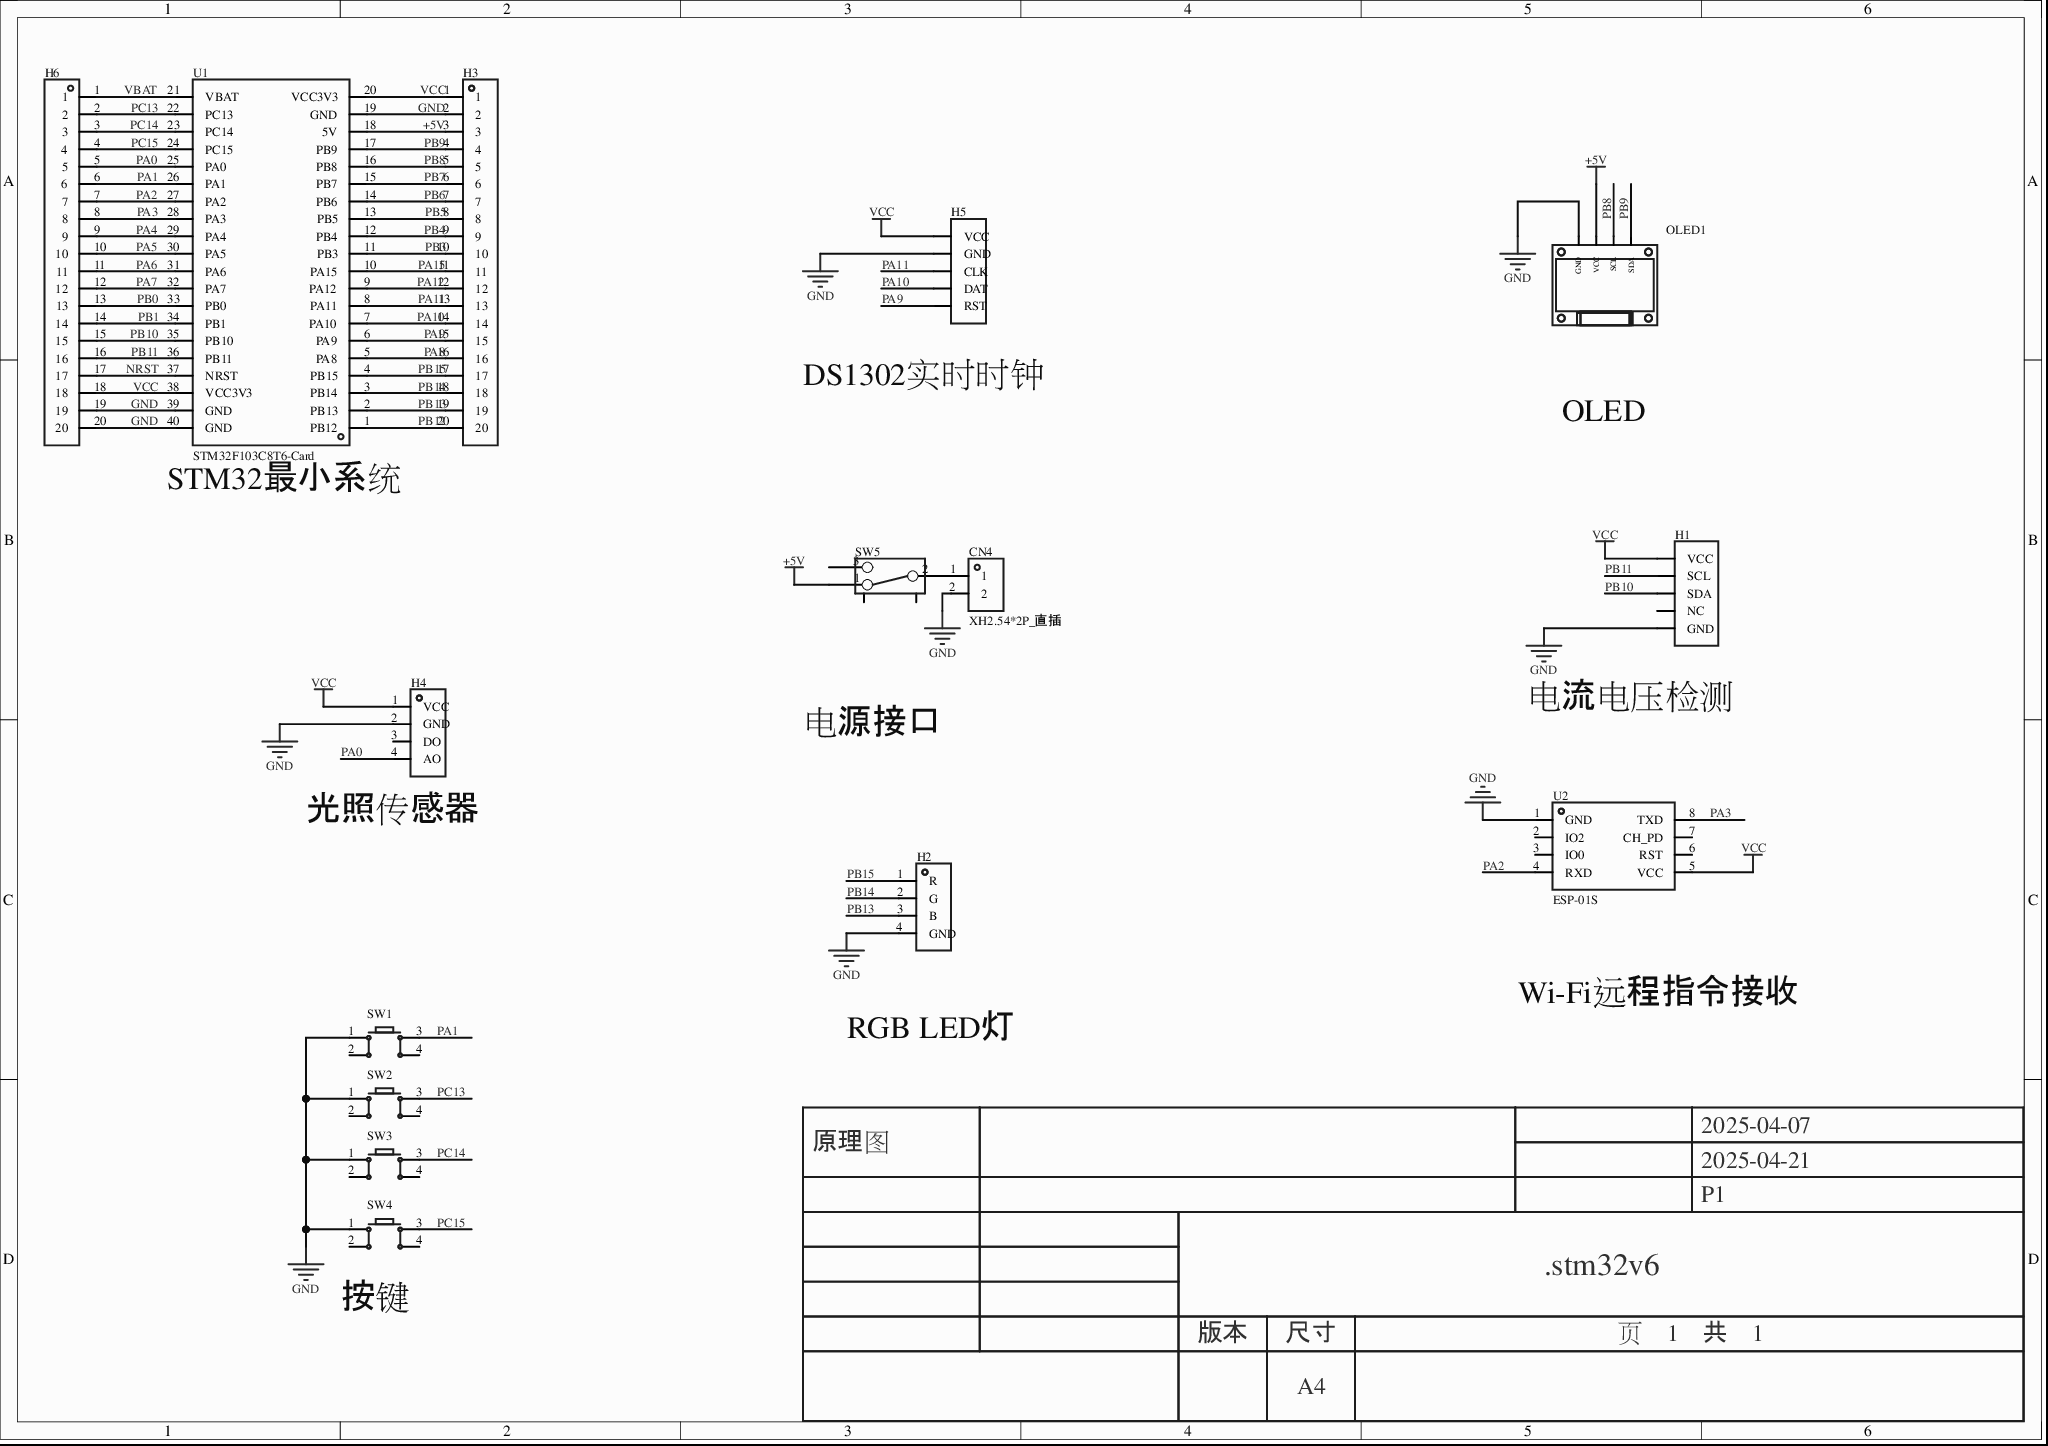
[diagram p0: MISC51840-3.schdoc]
# Altium project MISC51840-2.PrjPcb
1 sheet, 15 parts. Net scope: global (net labels, ports and power ports of the same name join across sheets).
Board file: MISC51840.pcbdoc

## Sheet MISC51840-3.schdoc
size 297 x 209 mm; Version: V1.0; @Project Name: MISC51840; @Page Count: 1; @Update Date: 2026-05-15; @Create Date: 2026-05-15; @Schematic Name: MISC51840; @Page No: 1; @Create Time: 23:22:16; @Update Time: 17:32:40; @Board Name: MISC51840

### Parts
CN4  XH2.54*2P_直插  [CONN-TH_2P-P2.50-XH2.54-2P]
H1  (no value)  [HDR-TH_5P-P2.54-V-F]
H2  (no value)  [HDR-TH_4P-P2.54-V-F]
H3  (no value)  [HDR-TH_20P-P2.54-V-M-1]
H4  (no value)  [HDR-TH_4P-P2.54-V-F]
H5  (no value)  [HDR-TH_5P-P2.54-V-F]
H6  (no value)  [HDR-TH_20P-P2.54-V-M-1]
OLED1  (no value)  [0.96OLED_4P]
SW1  (no value)  [SW-TH_4P-L6.0-W6.0-P4.50-LS6.5]
SW2  (no value)  [SW-TH_4P-L6.0-W6.0-P4.50-LS6.5]
SW3  (no value)  [SW-TH_4P-L6.0-W6.0-P4.50-LS6.5]
SW4  (no value)  [SW-TH_4P-L6.0-W6.0-P4.50-LS6.5]
SW5  (no value)  [拨动开关]
U1  STM32F103C8T6-Card  [CONN-TH_L53.3-W22.9_STM32F103C8T6-CARD]
U2  ESP-01S  [WIFIM-TH_ESP-01S]

### Nets
+5V: H3.3 OLED1.2(VCC) SW5.1 U1.18(5V)
GND: CN4.2 H1.5(GND) H2.4(GND) H3.2 H4.2(GND) H5.2(GND) H6.19 H6.20 OLED1.1(GND) SW1.1 SW2.1 SW3.1 SW4.1 U1.19(GND) U1.39(GND) U1.40(GND) U2.1(GND)
VCC: H1.1(VCC) H3.1 H4.1(VCC) H5.1(VCC) H6.18 U1.20(VCC3V3) U1.38(VCC3V3) U2.5(VCC)
NRST: H6.17 U1.37(NRST)
PA0: H4.4(AO) H6.5 U1.25(PA0)
PA1: H6.6 SW1.3 U1.26(PA1)
PA2: H6.7 U1.27(PA2) U2.4(RXD)
PA3: H6.8 U1.28(PA3) U2.8(TXD)
PA4: H6.9 U1.29(PA4)
PA5: H6.10 U1.30(PA5)
PA6: H6.11 U1.31(PA6)
PA7: H6.12 U1.32(PA7)
PA8: H3.16 U1.5(PA8)
PA9: H3.15 H5.5(RST) U1.6(PA9)
PA10: H3.14 H5.4(DAT) U1.7(PA10)
PA11: H3.13 H5.3(CLK) U1.8(PA11)
PA12: H3.12 U1.9(PA12)
PA15: H3.11 U1.10(PA15)
PB0: H6.13 U1.33(PB0)
PB1: H6.14 U1.34(PB1)
PB3: H3.10 U1.11(PB3)
PB4: H3.9 U1.12(PB4)
PB5: H3.8 U1.13(PB5)
PB6: H3.7 U1.14(PB6)
PB7: H3.6 U1.15(PB7)
PB8: H3.5 OLED1.3(SCL) U1.16(PB8)
PB9: H3.4 OLED1.4(SDA) U1.17(PB9)
PB10: H1.3(SDA) H6.15 U1.35(PB10)
PB11: H1.2(SCL) H6.16 U1.36(PB11)
PB12: H3.20 U1.1(PB12)
PB13: H2.3(B) H3.19 U1.2(PB13)
PB14: H2.2(G) H3.18 U1.3(PB14)
PB15: H2.1(R) H3.17 U1.4(PB15)
PC13: H6.2 SW2.3 U1.22(PC13)
PC14: H6.3 SW3.3 U1.23(PC14)
PC15: H6.4 SW4.3 U1.24(PC15)
VBAT: H6.1 U1.21(VBAT)
NetCN4_1: CN4.1 SW5.2

Not connected (* = marked no-connect by the designer): H1 4(NC); H4 3(DO); SW1 2 4; SW2 2 4; SW3 2 4; SW4 2 4; SW5 3 4 5; U2 2(IO2)* 3(IO0)* 6(RST)* 7(CH_PD)*

### Notes on the sheet
- (near H5) DS1302实时时钟
- OLED
- (near U1) STM32最小系统
- 电源接口
- 电流电压检测
- (near H4) 光照传感器
- RGB LED灯
- Wi-Fi远程指令接收
- (near SW4) 按键
- 2025-04-07
- 原理图
- 2025-04-21
- P1
- .stm32v6
- 版本
- 尺寸
- A4
- 页    1    共    1

### Library data of the parts
CN4 = XH2.54*2P_直插: 3D Model: 325c595e30db4df8abe76612dd40b0fa0819f05c4eef4c71ace90d822a990e87; 3D Model Transform: 295.275,228.346,0,180,0,0,-0.002,-20.079,-137.795; AddInBom: yes; Symbol: XH2.54*2P_直插; Device: XH2.54*2P_直插; LCSC Part Name: XH2.54*2P_直插; Supplier Part: C9900008615; Manufacturer Part: XH2.54*2P_直插; Supplier Footprint: XH2.54_2P; JLCPCB Part Class: Extended Part; Supplier: LCSC; ConvertToPcb: yes; FootprintName: CONN-TH_2P-P2.50-XH2.54-2P; ModelName: CONN-TH_2P-P2.50-XH2.54-2P
H1 = HDR-F_2.54_1x5P: Symbol: Header-Female-2.54_1x5_2; 3D Model: f49cb6116a3d45e5a64915bf3e00773f; 3D Model Transform: 519.684,98.464,0,0,0,0,0,0,-124.016; ConvertToPcb: yes; Device: HDR-F_2.54_1x5P; Supplier Part: C50950; Supplier Footprint: 插件; AddInBom: yes; FootprintName: HDR-TH_5P-P2.54-V-F; ModelName: HDR-TH_5P-P2.54-V-F
H2 = HDR-F_2.54_1x4P: Symbol: 2.54-1*4P母_2; ConvertToPcb: yes; ModelId: d187812051054f85879fcaa51a310d8e0819f05c4eef4c71ace90d822a990e87; ModelTransform: 419.6842,98.464,0,0,0,0,0,0,-118.11; Device: HDR-F_2.54_1x4P; AddInBom: yes; SupplierPart: C2718488; Supplier Footprint: 插件; FootprintName: HDR-TH_4P-P2.54-V-F; ModelName: HDR-TH_4P-P2.54-V-F
H3 H6 = HDR-M_2.54_1x20P: 间距:2.54mm;总PIN位数:20;排数:1;插针结构:-;行距:-;安装类型:直插;圆针/方针:-;额定电流:-;额定电压:-;配合针长度:-;塑高:-;触头材质:黄铜;触头镀层:-;颜色:黑色;; Symbol: HDR_2.54-1x20P; ConvertToPcb: yes; ModelId: f68709be121d406db68b06f32a5953890819f05c4eef4c71ace90d822a990e87; ModelName: HDR-M-2.54_1x20; ModelTransform: 1999.996,100,0,0,0,0,0,0,-118.11; Device: HDR-M_2.54_1x20P; AddInBom: yes; SupplierPart: C50981; Supplier Footprint: 插件; FootprintName: HDR-TH_20P-P2.54-V-M-1
H4 = HDR-F_2.54_1x4P: Symbol: 2.54-1*4P母_1; ConvertToPcb: yes; ModelId: d187812051054f85879fcaa51a310d8e0819f05c4eef4c71ace90d822a990e87; ModelTransform: 419.6842,98.464,0,0,0,0,0,0,-118.11; Device: HDR-F_2.54_1x4P; FootprintName: HDR-TH_4P-P2.54-V-F; AddInBom: yes; SupplierPart: C2718488; Supplier Footprint: 插件; ModelName: HDR-TH_4P-P2.54-V-F
H5 = HDR-F_2.54_1x5P: Symbol: Header-Female-2.54_1x5_1; ConvertToPcb: yes; ModelId: f49cb6116a3d45e5a64915bf3e00773f; ModelTransform: 519.684,98.464,0,0,0,0,0,0,-124.016; Device: HDR-F_2.54_1x5P; AddInBom: yes; SupplierPart: C50950; Supplier Footprint: 插件; FootprintName: HDR-TH_5P-P2.54-V-F; ModelName: HDR-TH_5P-P2.54-V-F
OLED1 = 0.96OLED模块_4P: ConvertToPcb: yes; ModelId: 79c000fdb68d45a296c2e9bedf4f9055; ModelTransform: 1393.69792,1318.895,0,0,0,0,0,-560.079,-137.795; Device: 0.96OLED模块_4P; Symbol: 0.96OLED模块_4P; FootprintName: 0.96OLED_4P; AddInBom: yes; Supplier Footprint: 插件; ModelName: 0.96OLED_4P
SW1-SW4 = Key_TH_6x6x6: 触点电流:50mA;额定电压(DC):12V;绝缘电阻:100MΩ;电路结构:单刀单掷;安装方式:直插;按钮形状:圆形按钮;按钮/盖帽颜色:黑色;作用力:260gf@±30gf;工作温度:-25℃~+70℃;引脚样式:PC引脚;开关长度:6mm;开关宽度:6mm;开关高度:6mm;带支架:否;; Symbol: 轻触按键; AddInBom: yes; ModelId: 20eee248bc684ccd8cbdbb1d0d91ec6f0819f05c4eef4c71ace90d822a990e87; ModelName: SW-TH_4P-L6.0-W6.0-H5.0-LS6.5-P4.50; ModelTransform: 236.22,323.03,0,90,0,0,0,0,-137.795; Device: Key_TH_6x6x6; FootprintName: SW-TH_4P-L6.0-W6.0-P4.50-LS6.5; ConvertToPcb: yes; Supplier Footprint: 插件
SW5 = 拨动开关_正: 3D Model: 4321fe59a4074cbfb4989553f297c68f0819f05c4eef4c71ace90d822a990e87; 3D Model Transform: 370.09,208.7,472.35,0,0,0,0,0,-110; ConvertToPcb: yes; ModelName: SW-TH_SS-12D02-VG4; Symbol: 拨动开关; Device: 拨动开关_正; Supplier Footprint: 插件; AddInBom: yes; FootprintName: 拨动开关
U1 = STM32F103C8T6-Card: AddInBom: yes; Device: STM32F103C8T6-Card; Symbol: STM32F103C8T6-CARD; FootprintName: CONN-TH_L53.3-W22.9_STM32F103C8T6-CARD; LCSC Part Name: STM32F103C8T6-Card; SupplierPart: C9900077949; ManufacturerPart: STM32F103C8T6-Card; Supplier Footprint: 插件; Supplier: LCSC; ConvertToPcb: yes
U2 = ESP-01S_C111009: 3D Model: eb7175da78ae48b3b1568cfe3027405f0819f05c4eef4c71ace90d822a990e87; 3D Model Transform: 582.676,976.37608,0,0,0,0,0,388.346,-118.11; AddInBom: yes; Symbol: ESP-01S; Device: ESP-01S_C111009; LCSC Part Name: ESP-01S; Supplier Part: C111009; Manufacturer Part: ESP-01S; Supplier Footprint: -; JLCPCB Part Class: Extended Part; Supplier: LCSC; ConvertToPcb: yes; FootprintName: WIFIM-TH_ESP-01S; ModelName: WIFIM-TH_ESP-01S